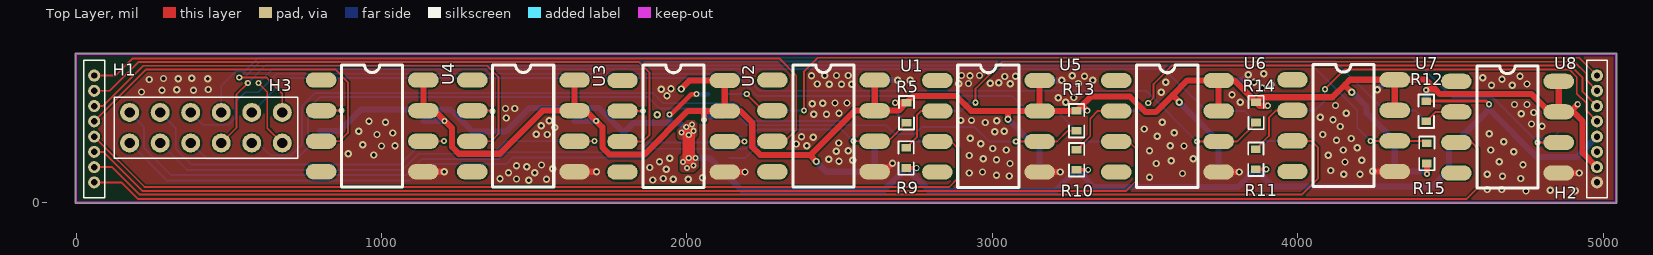
[diagram p0: Top Layer view]
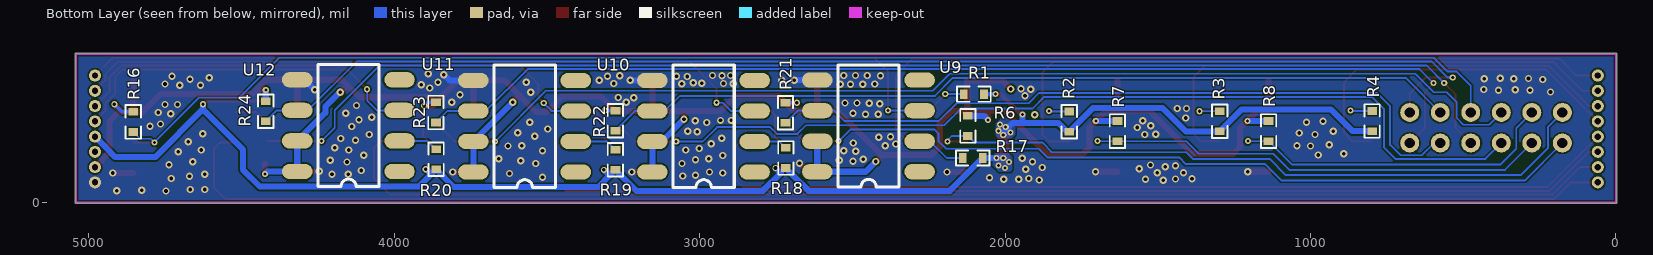
[diagram p1: Bottom Layer view, seen from below]
# Altium PCB MISC82214.PcbDoc
Units mil, origin at the board's own origin, x right, y up, seen from the top; angles counter-clockwise.
Board outline 5048.08 x 492.03 mil, 2 copper layers (Top Layer, Bottom Layer); 39 components, 39 nets, 172 pads, 235 vias.

## Layer stack, top to bottom (the 12.6 mil dielectric is the usual default, probably not edited)
Top Layer: signal copper 1.4
Dielectric: dielectric 12.6, FR-4, Dk 4.8
Bottom Layer: signal copper 1.4

## Board outline
0,-3.02 cw(c0,0) -3.02,0 -3.02,485.43 cw(c-0.06,486) -0.06,489.02 5039.31,489.02 cw(c5039.31,486) 5040.66,488.7 cw(c5042,486) 5045.02,486 5045.02,0 cw(c5042,0) 5040.66,-2.7 cw(c5039.31,0) 5039.31,-3.02

## Design rules (kind name [scope] priority, off if disabled: settings)
Clearance [All] p1: gap=6
FabricationTestPointUsage TestPointUsage [All] p1: valid=0 allowmultiple=FALSE
FabricationTestpoint Testpoint [(IsPad And (OnTopLayer Or OnBottomLayer))] p1: side=3 testpointundercomponent=TRUE minsize=40 maxsize=100 preferedsize=60 minholesize=0 maxholesize=40 preferedholesize=32 testpointgrid=1 allowsidetop=TRUE allowsidebottom=TRUE usegrid=TRUE gridtolerance=0.01
HoleSize [All] p1: absolutevalues=TRUE maxlimit=100 minlimit=8 maxpercent=80.000 minpercent=20.000
PlaneClearance [All] p1: clearance=30
PlaneConnect [All] p1: planeconnectstyle=Direct reliefexpansion=20 reliefentries=4 reliefconductorwidth=10 reliefairgap=10
PolygonConnect [All] p1: connectstyle=Direct reliefconductorwidth=6 reliefentries=4 polygonreliefangle="90 Angle"
RoutingVias [All] p1: holewidth=12 width=24 viastyle="Through Hole" minholewidth=10 minwidth=20 maxholewidth=12 maxwidth=24
SilkscreenOverComponentPads [IsPad] p1: minsilkscreentomaskgap=10
SolderMaskExpansion [All] p1: expansion=4
Width [All] p1: maxlimit=40 minlimit=6 preferedwidth=6 minimp=50.000000 maximp=50.000000 favimp=50.000000
22 further rules are at their usual default settings.

## Components (designator, comment, footprint, x,y, rotation, side; value= is the part's Value field where it differs from the comment)
H1 "Header8" PinHeader8_1.27mm 59,416 r270 top locked
H2 "Header8" PinHeader8_1.27mm 4980.26,416 r270 top locked
H3 "Header6*2" PinHeader6*2_2.54mm 175,195 r0 top
R1 "470R" 0603 2135,355 r180 bottom
R2 "470R" 0603 1790,298 r270 bottom
R3 "470R" 0603 1297,299 r270 bottom
R4 "470R" 0603 798,300 r270 bottom
R5 "4.7k" 0603 2719,327 r270 top
R6 "4.7k" 0603 2122,284 r270 bottom
R7 "4.7k" 0603 1632,267 r270 bottom
R8 "4.7k" 0603 1137,267 r270 bottom
R9 "470R" 0603 2718,179 r270 top
R10 "470R" 0603 3276,173 r270 top
R11 "470R" 0603 3863,175 r270 top
R12 "470R" 0603 4421,266 r90 top
R13 "4.7k" 0603 3276,301 r270 top
R14 "4.7k" 0603 3864,328 r270 top
R15 "4.7k" 0603 4423,128 r90 top
R16 "4.7k" 0603 4855,297 r270 bottom
R17 "470R" 0603 2139,146 r180 bottom
R18 "470R" 0603 2718,179 r270 bottom
R19 "470R" 0603 3276,173 r270 bottom
R20 "470R" 0603 3863,175 r270 bottom
R21 "4.7k" 0603 2719,327 r270 bottom
R22 "4.7k" 0603 3276,301 r270 bottom
R23 "4.7k" 0603 3864,328 r270 bottom
R24 "4.7k" 0603 4421,332 r270 bottom
U1 "6N137" 6N137_SMD 2280,401 r0 top
U2 "6N137" 6N137_SMD 1789,400 r0 top
U3 "6N137" 6N137_SMD 1297,401 r0 top
U4 "6N137" 6N137_SMD 802,401 r0 top
U5 "6N137" 6N137_SMD 2820,400 r0 top
U6 "6N137" 6N137_SMD 3406,400 r0 top
U7 "6N137" 6N137_SMD 3983,402 r0 top
U8 "6N137" 6N137_SMD 4520,397 r0 top
U9 "6N137" 6N137_SMD 2280,101 r0 bottom
U10 "6N137" 6N137_SMD 2820,100 r0 bottom
U11 "6N137" 6N137_SMD 3406,100 r0 bottom
U12 "6N137" 6N137_SMD 3983,102 r0 bottom

## Footprints (in the part's own frame and the unit in brackets; to place one, negate y for a bottom-side part, rotate by r counter-clockwise, add the part's x,y. Pads: shape width x height; smd on the part's side, far side on the other; paste and mask are expansions set on the pad)
6N137_SMD [mil]
  oval 100x50 smd: 1(0,0) 2(0,-100) 3(0,-200) 4(0,-300) 5(335,-300) 6(335,-200) 7(335,-100) 8(335,0)
  silkscreen extent 67,-350 267,50
0603 [mil]
  rect 25x32 smd: 1(0,0) 2(66,0)
  silkscreen extent -22,-25 88,25
PinHeader6*2_2.54mm [mil]
  round 62 hole 34: 1(0,0) 2(0,100) 3(100,0) 4(100,100) 5(200,0) 6(200,100) 7(300,0) 8(300,100) 9(400,0) 10(400,100) 11(500,0) 12(500,100)
  silkscreen extent -50,-50 550,150
PinHeader8_1.27mm [mm]
  round 1 hole 0.533: 1(0,0) 2(1.27,0) 3(2.54,0) 4(3.81,0) 5(5.08,0) 6(6.35,0) 7(7.62,0) 8(8.89,0)
  silkscreen extent -1.27,-0.87 10.16,0.87

## Part data
R1 R2 R3 R4 R5 R6 R7 R8 R9 R10 R11 R12 R13 R14 R15 R16 R17 R18 R19 R20 R21 R22 R23 R24: library part RES
U1 U2 U3 U4 U5 U6 U7 U8 U9 U10 U11 U12: "High-speed optocoupler"

## Via types
v1: diameter 24, hole 12, Top Layer to Bottom Layer, 191 vias
v2: diameter 20, hole 10, Top Layer to Bottom Layer, 37 vias
v3: diameter 20, hole 12, Top Layer to Bottom Layer, 7 vias

## Nets (pads, with @x,y where several pads share a name; then routed paths per layer and width w, separated by ;. In a path a pad name is that pad's centre, name@x,y a point inside that pad or via, vN(x,y) a via of type N, cw(c..) or ccw(c..) an arc to the next point about the centre after c; other vN are vias at no path point)
+5V: H2.5 R1.2 R2.2 R3.2 R4.2 R9.2 R10.2 R11.2 R12.2 R17.2 R18.2 R19.2 R20.2 | length 5426.7
  Top Layer w10: R11.2 v3(3897,109) ; R12.2 4422,333 4616,333 v2(4627,322)
  Top Layer w12: R9.2 v3(2752,113) ; R10.2 v3(3314,107)
  Top Layer w15: v2(1943,288) 1947,288 2014,355 v2(2031,355)
  Top Layer w40: v2(2006,146) v2@2006,223
  Bottom Layer w15: v2(2031,355) R1.2
  Bottom Layer w20: R4.2 862,234 933,305 1225,305 R3.2 1408,233 1485,310 1712,310 R2.2 1797,232 1825,260 1946,260 ; v2(1943,288) 1943,263 1946,260 ; v2(2006,146) R17.2 2181,38 2643,38 2690,85 R18.2 ; v2(2006,221) 2006,223 2005,224 2005,229 2006,230 1976,260 1946,260 ; v3@2751,112 2735.5,96.5 2734.5,96.5 2793,38 3207,38 R19.2 3292.5,90.5 ; v3@3313,106 3297.5,90.5 3292.5,90.5 ; v3(3897,109) 3896,109 3879.5,92.5 ; v2(4627,322) 4627,305 ; H2.5 4979.79,216 4944.57,180.78 4944.57,180.31 4913.26,149 4783,149 4627,305 ; 3292.5,90.5 3332,51 3805,51 R20.2 3879.5,92.5 ; 3879.5,92.5 3920,52 4440,52 4496,108 4496,174 4627,305
  other v2: 2000,113 2022,121 1987,133 2028,146 1982,230 2021,235 1998,247 2017,256
+5V_EXT: H2.7 R5.1 R6.1 R7.1 R8.1 R13.1 R14.1 R15.1 R16.1 R21.1 R22.1 R23.1 R24.1 U1.7 U1.8 U2.7 U2.8 U3.7 U3.8 U4.7 U4.8 U5.7 U5.8 U6.7 U6.8 U7.7 U7.8 U8.7 U8.8 U9.7 U9.8 U10.7 U10.8 U11.7 U11.8 U12.7 U12.8 | length 7616.8
  Top Layer w20: U4.8 U4.7 1174,301 1231,244 1231,182 1253,160 1387,160 1528,301 1669,301 v2(1703,267) 1723,247 1723,181 1747,157 1860,157 2003,300 2062,300 ; U3.7 U3.8 ; v1(1981,372) 2009,400 U2.8 U2.7 ; v2@2056,274 2056,294 2062,300 ; 2402,156 2240,156 2214,182 2214,261 2175,300 U2.7 ; v1(2423.75,134.25) 2403.5,154.5 2550,301 U1.7 ; U1.8 U1.7 ; v3@2684,327 R5.1 ; v1(3051.68,273.32) 3052,273.65 3052,300 ; U5.8 U5.7 ; v3@3310,302 3296.5,315.5 3290.5,315.5 ; v1@3612,331 3591,352 ; U6.7 U6.8 ; U6.8@3749,400 U6.8 ; 3792,400 R14.1 ; v3(3902,317) 3875,317 R14.1 ; v1(4177,361) 4155,383 4155,386 ; U7.7 U7.8 ; v2(4421,369) 4422.5,370.5 4450.5,370.5 ; v2(4423,94) R15.1 ; U8.8 U8.7 ; U8.7@4902,297 4933,266 4933,162.79 4979.79,116 H2.7 ; v3@4916,320 4893,297 U8.7 ; 2062,300 U2.7 ; U1.7 2693,301 R5.1 ; R5.1 2741,349 2882,349 2931,300 3052,300 ; 3052,300 U5.7 ; U5.7 3275,300 R13.1 3290.5,315.5 ; 3290.5,315.5 3322,347 3451,347 3502,296 3535,296 3591,352 ; 3591,352 3639,400 U6.8 ; R14.1 3881,345 4114,345 4155,386 ; 4155,386 4171,402 U7.8 ; U7.8 4419,402 4450.5,370.5 ; 4450.5,370.5 4466,355 4766,355 4824,297 U8.7
  Bottom Layer w12: v3(2682,327) R21.1 ; R22.1 v3(3311,301) ; R23.1 3891,328 v3(3902,317) ; R16.1 4892,297 v3(4917,322)
  Bottom Layer w20: R8.1 v2(1206.69,267) ; R7.1 v2(1703,267) ; v2(2056,271) 2069,284 R6.1 ; v1(2423.75,134.25) 2457,101 U9.8 U9.7 ; v1(3051.68,273.32) 3125,200 U10.7 U10.8 ; v1(3612,329) U11.7 U11.8 ; v1@4177,363 4226,314 4226,294 U12.7 U12.8 4415,102 v2(4423,94) ; R24.1 v2(4421,369)
GND_EXT: H2.8 U1.5 U2.5 U3.5 U4.5 U5.5 U6.5 U7.5 U8.5 U9.5 U10.5 U11.5 U12.5 | length 874.6
  Top Layer w20: U4.5 v1(1205,101) ; U3.5 v1(1704,101) ; U2.5 v1(2190,100) ; U1.5 2645,101 2664,120 v1(2673,129) ; U5.5 3209,100 v1(3223,100) ; U6.5 v1(3809,100) ; v1(4246,102) U7.5 ; U8.5 v1(4922,97)
  Bottom Layer w20: U9.5 v1(2690,401) ; U10.5 v1(3227,400) ; v1@3222,99 v1(3223,100) ; U11.5 3819,400 v1(3838,419) ; v1(4261,369) 4294,402 U12.5
  other v1: 4748,38 4909,39 4827,40 4621,43 4668,43 1482,73 1888,74 1540,76 1955,76 2004,76 1442,77 1388,78 1922,79 4731,79 2051,81 3515,83 4671,86 3056,87 3014,89 4151,93 4204,93 4621,93 3623,95 2925,97 1416,98 1502,98 2968,100 4108,105 1932,109 1561,111 1878,115 1475,117 1442,121 1524,123 4738,124 3058,128 3537,128 4155,133 1910,134 4660,134 2498,135 3586,137 2543,139 4210,139 3014,140 2464,142 2970,143 3658,144 1944,145 2925,154 4100,155 975,156 891,160 4708,166 2489,168 2528,170 3515,170 3046,172 4149,172 4632,172 3001,177 4195,180 1000,185 3628,185 1044,186 2392,186 3583,186 938,189 2358,192 2962,193 2497,195 4675,199 4127,204 4175,210 2928,211 2414,214 2375,215 3540,217 985,223 1543,223 4082,223 1507,224 4627,225 1037,228 3596,229 3008,232 3039,233 925,234 3498,241 1567,246 4140,249 4800,250 1523,251 4766,257 2977,262 1013,263 3557,263 959,266 1549,268 3015,268 2897,269 2932,269 4116,271 1408,277 4074,279 2415,289 2457,289 4732,291 4159,292 2498,293 4773,295 1406,308 1436,308 4124,318 4710,321 4751,321 2410,324 2445,325 2485,326 2524,326 3241,328 3812,329 3216,343 3267,344 1935,350 3785,353 3553,361 214,362 281,368 384,368 329,369 433,370 1916,371 1948,373 3884,375 4635,384 4703,384 3912,386 2466,387 2506,387 2540,387 2427,388 4751,388 2890,389 3059,389 2922,390 3282,390 2993,391 3021,392 3568,394 3857,394 3329,400 2731,401 239,403 4669,404 334,405 431,405 286,406 379,407 4606,409 3041,413 3076,414 3302,414 4728,414 2408,415 2927,415 3262,415 2451,416 2490,416 2528,416 2899,416 2958,416 3889,422
IN1: H1.1 U1.3 | length 2616.7
  Top Layer w6: H1.1 130,416 186,472 2302,472 2358,416 2358,238 2321,201 U1.3
IN2: H1.2 U2.3 | length 2173.3
  Top Layer w6: H1.2 110,366 204,460 1844,460 1877,427 1877,221 1856,200 U2.3
IN3: H1.3 U3.3 | length 1675.9
  Top Layer w6: H1.3 87,316 219,448 1346,448 1383,411 1383,225 1359,201 U3.3
IN4: H1.4 U4.3 | length 1184
  Top Layer w6: H1.4 229,436 848,436 890,394 890,228 863,201 U4.3
IN5: H1.5 U5.3 | length 3121.1
  Top Layer w6: H1.5 224,51 869,51 ; 907,51 869,51 ; U5.3 2865,200 2887,178 2887,79 2859,51 869,51
IN6: H1.6 U6.3 | length 3658.4
  Top Layer w6: H1.6 89,166 217,38 3438,38 3470.68,70.68 3470.68,176.32 3447,200 U6.3
IN7: H1.7 U7.3 | length 4260.8
  Top Layer w6: H1.7 118,116 208,26 4014,26 4067,79 4067,179 4044,202 U7.3
IN8: H1.8 U8.3 | length 4775.8
  Top Layer w6: H1.8 148,66 202,12 4554,12 4590.32,48.32 4590.32,176.68 4570,197 U8.3
IN9: H2.1 U9.3 | length 2870.3
  Top Layer w6: v2(2383,301) 2383,428 2429,474 4922.26,474 H2.1
  Bottom Layer w6: U9.3 v2(2383,301)
IN10: H2.2 U10.3 | length 2305.4
  Top Layer w6: v2(2945,327) 2945,373 3033,461 4906,461 4946.01,420.99 4946.01,400.25 H2.2
  Bottom Layer w6: U10.3 2898,300 2925,327 v2(2945,327)
IN11: H2.3 U11.3 | length 1744.3
  Top Layer w6: v2(3510.73,325.73) 3528,343 3528,388 3589,449 4893.05,449 4933,409.05 4933,363.26 H2.3
  Bottom Layer w6: U11.3 3485,300 v2(3510.73,325.73)
IN12: H2.4 U12.3 | length 1191
  Top Layer w6: v2(4089,371) 4154,436 4625.03,436 4800,436 4889.08,436 4914,411.08 4914,357 4946.01,324.99 4946.01,300.25 H2.4
  Bottom Layer w6: U12.3 4057,302 4089,334 v2(4089,371)
NetR1_1: R1.1 U1.2 | length 167.4
  Top Layer w6: v2(2196,355) 2250,301 U1.2
  Bottom Layer w6: R1.1 v2(2196,355)
NetR2_1: R2.1 U2.2 | length 133.8
  Top Layer w6: U2.2 v2(1856,300)
  Bottom Layer w6: R2.1 1854,298 v2(1856,300)
NetR3_1: R3.1 U3.2 | length 134.8
  Top Layer w6: U3.2 1362,301 v2(1364,299)
  Bottom Layer w6: R3.1 v2(1364,299)
NetR4_1: R4.1 U4.2 | length 138.4
  Top Layer w6: U4.2 v2(869,301)
  Bottom Layer w6: R4.1 868,300 v2(869,301)
NetR9_1: R9.1 U5.2 | length 194.3
  Top Layer w6: R9.1 2741.5,202.5 2744,205 2753,214 2753,286 2767,300 U5.2
NetR10_1: R10.1 U6.2 | length 216
  Top Layer w6: R10.1 3321,218 3321,275 3346,300 U6.2
NetR11_1: R11.1 U7.2 | length 207.8
  Top Layer w6: R11.1 3906,218 3906,278 3930,302 U7.2
NetR12_1: R12.1 U8.2 | length 111.8
  Top Layer w6: R12.1 4452,297 U8.2
NetR17_1: R17.1 U9.2 | length 163.8
  Bottom Layer w6: R17.1 2191,146 2246,201 U9.2
NetR18_1: R18.1 U10.2 | length 110.7
  Bottom Layer w6: R18.1 2739,200 U10.2
NetR19_1: R19.1 U11.2 | length 141.2
  Bottom Layer w6: R19.1 3303,200 U11.2
NetR20_1: R20.1 U12.2 | length 131.2
  Bottom Layer w6: R20.1 3866,175 3893,202 U12.2
OUT1: H3.1 R5.2 U1.6 | length 2719.4
  Top Layer w6: v2(2545,201) U1.6 2659,201 R5.2
  Bottom Layer w6: H3.1 298,72 1094,72 1148,126 1408,126 1430,148 1862,148 1890,176 2193,176 2218,201 2218,226 2231,239 2507,239 v2(2545,201)
OUT2: H3.2 R6.2 U2.6 | length 2270.2
  Top Layer w6: U2.6 v2(2188,200)
  Bottom Layer w6: H3.2 222,248 222,180 312,90 1081,90 1134,143 1385,143 1407,165 1847,165 1879,197 2101,197 R6.2 2174,218 2192,200 v2(2188,200)
OUT3: H3.3 R7.2 U3.6 | length 1562.4
  Top Layer w6: U3.6 v2(1697,201)
  Bottom Layer w6: H3.3 363,107 1069,107 1122,160 1366,160 1407,201 R7.2 v2(1697,201)
OUT4: H3.4 R8.2 U4.6 | length 1139.7
  Top Layer w6: U4.6 v2(1205,201)
  Bottom Layer w6: H3.4 326,244 326,176 377,125 1061,125 R8.2 v2(1205,201)
OUT5: H3.5 R13.2 U5.6 | length 3173
  Top Layer w6: v2(3077,200) U5.6 3212,200 3247,235 R13.2
  Bottom Layer w6: H3.5 427,143 722,143 759,180 759,305 800,346 1872,346 1910,308 2144,308 2199,253 2652,253 2680,225 2747,225 2769,247 2943,247 2990,200 v2(3077,200)
OUT6: H3.6 R14.2 U6.6 | length 3722.8
  Top Layer w6: v2(3670,200) U6.6 3802,200 R14.2
  Bottom Layer w6: H3.6 415,255 499,255 521,277 521,329 553,361 596,361 657,422 2181,422 2237,366 3504,366 v2(3670,200)
OUT7: H3.7 R15.2 U7.6 | length 4244.8
  Top Layer w6: H3.7 525,245 525,354 v2(562,391) ; v2(4238,202) U7.6 R15.2@4415,202
  Bottom Layer w6: v2(562,391) 620,449 3614.7,449 3710,449 4048,449 4195,302 4195,245 v2(4238,202)
OUT8: H3.8 R16.2 U8.6 | length 4703.5
  Top Layer w6: v2(4786,197) U8.6
  Bottom Layer w6: H3.8 475,383 521,429 551,429 596,474 4377,474 4508,343 4640,343 v2(4786,197) 4798,209 4833,209 R16.2
OUT9: H3.9 R21.2 U9.6 | length 2387.6
  Bottom Layer w6: H3.9 595,195 635,155 705,155 739,189 739,315 783,359 1889,359 1923,325 2159,325 2217,267 2526,267 2560,301 U9.6 2679,301 R21.2
OUT10: H3.10 R22.2 U10.6 | length 2819.5
  Bottom Layer w6: H3.10 688,408 2171,408 2230,349 3065,349 3114,300 U10.6 3211,300 R22.2
OUT11: H3.11 R23.2 U11.6 | length 3586.8
  Top Layer w6: v2(597,391) 626,362 626,244 H3.11
  Bottom Layer w6: v2(597,391) 643,437 3563,437 3700,300 U11.6 3826,300 R23.2
OUT12: H3.12 R24.2 U12.6 | length 4215.5
  Top Layer w6: v2(534,409) 535,410 622,410 675,357 H3.12
  Bottom Layer w6: v2(534,409) 550,409 603,462 4123,462 4283,302 U12.6 4385,302 R24.2
pads on no net: H2.6 U1.1 U1.4 U2.1 U2.4 U3.1 U3.4 U4.1 U4.4 U5.1 U5.4 U6.1 U6.4 U7.1 U7.4 U8.1 U8.4 U9.1 U9.4 U10.1 U10.4 U11.1 U11.4 U12.1 U12.4
copper on no net:
  other v1: 1903,288

## Polygon pours and split planes (outlines as drawn)
GND_EXT on Top Layer "Top Layer-No Net" (solid, remove dead copper): -97,522 -97,-144 -19,-222 29,-174 5182,-174 5182,471 5236,525 5059,702 2819,702 83,702 -97,522
+5V on Top Layer "Top Layer-No Net" (solid, remove dead copper): 1968,232 1968,217 1968,213 1972,209 1975,206 1995,206 2022,206 2028,212 2034,218 2034,234 2034,260 2026,268 2025,269 2019,269 1999,269 1982,252 1968,238 1968,231
+5V on Top Layer "Top Layer-No Net" (solid, remove dead copper): 1977,150 1977,106 1983,100 2005,100 2023,100 2032,109 2039,116 2039,146 2039,148 2030,157 2026,161 2006,161 1988,161 1977,150
GND_EXT on Bottom Layer "Top Layer-No Net" (solid, remove dead copper): -87,532 -60,505 -60,-49 5045,-49 5124,30 5144,50 5144,420 5144,529 5046,627 4970,551 -44,551 -68,551 -87,532
+5V on Bottom Layer "Top Layer-No Net" (solid, remove dead copper): 1967,251 1967,234 1967,222 1972,217 1979,210 1993,210 2021,210 2027,216 2031,220 2031,243 2031,258 2017,272 2012,277 2000,277 1993,277 1967,251
+5V on Bottom Layer "Top Layer-No Net" (solid, remove dead copper): 1976,150 1976,112 1976,108 1980,104 1983,101 2000,101 2020,101 2031,112 2040,121 2040,138 2040,154 2036,158 2032,162 2022,162 1988,162 1976,150

## Keep-outs
Keep-Out Layer:
  lines w6: -0.06,486 5039.32,486 ; 0,486 0,0 5039.32,0 ; 5042,0 5042,486